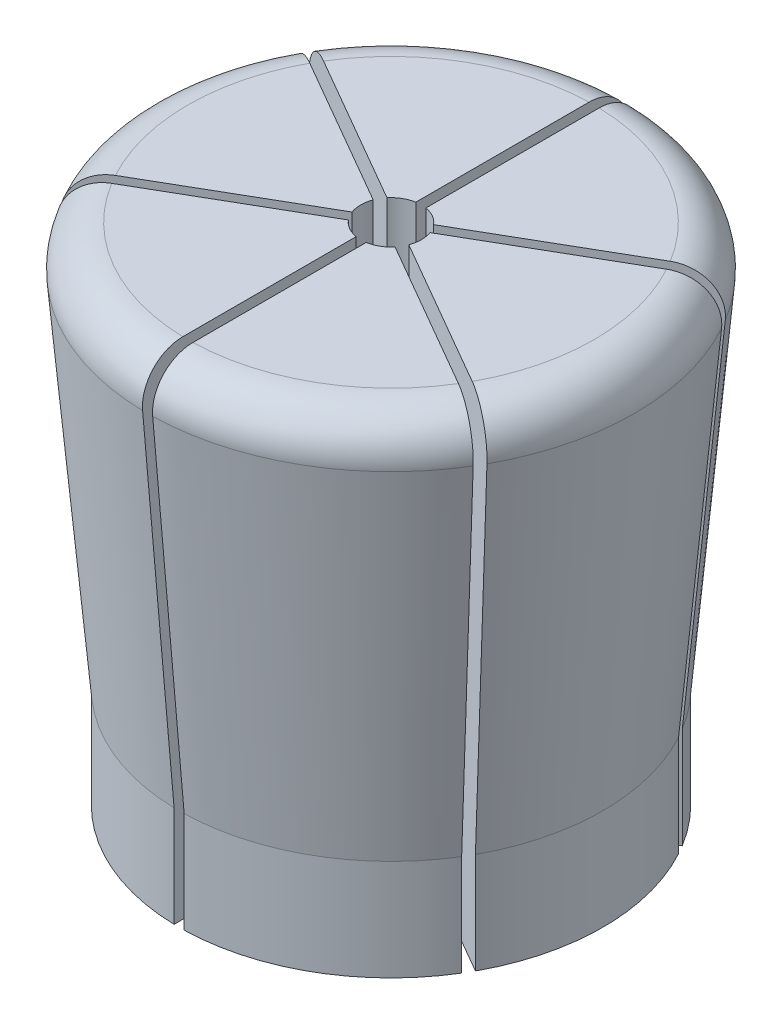
from build123d import *

# Parameters (mm, degrees)
SKETCH_2_R          = 1.5
CUT_EXTRUDE_1_DEPTH = 31.269333089
SKETCH_3_W          = 0.5
SKETCH_3_H          = 34.059940126
CUT_EXTRUDE_2_DEPTH = 31.269333089
CUT_EXTRUDE_3_DEPTH = 31.268300756
CUT_EXTRUDE_4_DEPTH = 31.268300756


with BuildPart() as part:
    # 草图1 → 旋转1 (revolve)
    with BuildSketch(Plane.XY, mode=Mode.PRIVATE) as revolve_1_sk:
        with BuildLine():
            Line((0, 25), (10.067156268, 25))
            ThreePointArc((10.067156268, 25), (11.541710942, 24.351180415), (12.059545665, 22.825688515))
            Line((12.059545665, 22.825688515), (10.5, 5))
            Line((10.5, 5), (10.5, 0))
            Line((10.5, 0), (0, 0))
            Line((0, 0), (0, 25))
        make_face()
    revolve(revolve_1_sk.sketch.rotate(Axis((0, 0, 0), (0, 1, 0)), 90), axis=Axis((0, 0, 0), (0, 1, 0)))

    # 草图2 → 切除-拉伸1 (cut, through all)
    with BuildSketch(Plane(origin=(0, 25, 0), x_dir=(1, 0, 0), z_dir=(0, 1, 0))):
        with Locations(Location((0, 0, 0), (0, 0, 270))):
            Circle(SKETCH_2_R)
    extrude(amount=-CUT_EXTRUDE_1_DEPTH, mode=Mode.SUBTRACT)

    # 草图3 → 切除-拉伸2 (cut, through all)
    with BuildSketch(Plane(origin=(0, 25, 0), x_dir=(1, 0, 0), z_dir=(0, 1, 0))):
        Rectangle(SKETCH_3_W, SKETCH_3_H)
    extrude(amount=-CUT_EXTRUDE_2_DEPTH, mode=Mode.SUBTRACT)


with BuildPart() as cut_extrude_2_piece_1:
    # of the separate pieces the step leaves, piece 1, a body of its own (cut_extrude_2_pieces)
    add(part.part.solids().sort_by_distance((0.25, 25, -10.064051636))[0])


with BuildPart() as cut_extrude_2_piece_2:
    # of the separate pieces the step leaves, piece 2, a body of its own (cut_extrude_2_pieces)
    add(part.part.solids().sort_by_distance((-0.25, 25, -10.064051636))[0])


with BuildPart() as cut_extrude_3_tool:
    # 草图4 → 切除-拉伸3 (new, through all)
    with BuildSketch(Plane(origin=(0, 25, 0), x_dir=(1, 0, 0), z_dir=(0, 1, 0))):
        Polygon((18.851057357, -11.172338174), (19.101057357, -10.739325472), (-18.851057357, 11.172338174), (-19.101057357, 10.739325472), align=None)
    extrude(amount=-CUT_EXTRUDE_3_DEPTH)


with BuildPart() as cut_extrude_2_piece_1_1:
    add(cut_extrude_2_piece_1.part)

    # 切除-拉伸3: cut by cut_extrude_3_tool
    add(cut_extrude_3_tool.part, mode=Mode.SUBTRACT)


with BuildPart() as cut_extrude_2_piece_2_1:
    add(cut_extrude_2_piece_2.part)

    # 切除-拉伸3: cut by cut_extrude_3_tool
    add(cut_extrude_3_tool.part, mode=Mode.SUBTRACT)


with BuildPart() as cut_extrude_3_piece_1:
    # of the separate pieces the step leaves, piece 1, a body of its own (cut_extrude_3_pieces)
    add(cut_extrude_2_piece_1_1.part.solids().sort_by_distance((0.25, 25, -10.064051636))[0])


with BuildPart() as cut_extrude_3_piece_2:
    # of the separate pieces the step leaves, piece 2, a body of its own (cut_extrude_3_pieces)
    add(cut_extrude_2_piece_1_1.part.solids().sort_by_distance((1.155868846, 25, 0.956016324))[0])


with BuildPart() as cut_extrude_3_piece_1_of_cut_extrude_2_p:
    # of the separate pieces the step leaves, piece 1, a body of its own (cut_extrude_3_pieces_of_cut_extrude_2_pi)
    add(cut_extrude_2_piece_2_1.part.solids().sort_by_distance((-8.840724382, 25, -4.815519467))[0])


with BuildPart() as cut_extrude_3_piece_2_of_cut_extrude_2_p:
    # of the separate pieces the step leaves, piece 2, a body of its own (cut_extrude_3_pieces_of_cut_extrude_2_pi)
    add(cut_extrude_2_piece_2_1.part.solids().sort_by_distance((-0.25, 25, -10.064051636))[0])


with BuildPart() as cut_extrude_4_tool:
    # 草图5 → 切除-拉伸4 (new, through all)
    with BuildSketch(Plane(origin=(0, 25, 0), x_dir=(1, 0, 0), z_dir=(0, 1, 0))):
        Polygon((-13.95064617, -7.765734187), (-13.70064617, -8.198746889), (13.95064617, 7.765734187), (13.70064617, 8.198746889), align=None)
    extrude(amount=-CUT_EXTRUDE_4_DEPTH)


with BuildPart() as cut_extrude_3_piece_1_1:
    add(cut_extrude_3_piece_1.part)

    # 切除-拉伸4: cut by cut_extrude_4_tool
    add(cut_extrude_4_tool.part, mode=Mode.SUBTRACT)


with BuildPart() as cut_extrude_3_piece_1_of_cut_extrude_2_p_1:
    add(cut_extrude_3_piece_1_of_cut_extrude_2_p.part)

    # 切除-拉伸4: cut by cut_extrude_4_tool
    add(cut_extrude_4_tool.part, mode=Mode.SUBTRACT)


with BuildPart() as cut_extrude_4_piece_1:
    # of the separate pieces the step leaves, piece 1, a body of its own (cut_extrude_4_pieces)
    add(cut_extrude_3_piece_1_1.part.solids().sort_by_distance((1.405868846, 25, -0.523003622))[0])


with BuildPart() as cut_extrude_4_piece_2:
    # of the separate pieces the step leaves, piece 2, a body of its own (cut_extrude_4_pieces)
    add(cut_extrude_3_piece_1_1.part.solids().sort_by_distance((0.25, 25, -10.064051636))[0])


with BuildPart() as cut_extrude_4_piece_1_of_cut_extrude_3_p:
    # of the separate pieces the step leaves, piece 1, a body of its own (cut_extrude_4_pieces_of_cut_extrude_3_pi)
    add(cut_extrude_3_piece_1_of_cut_extrude_2_p_1.part.solids().sort_by_distance((-8.840724382, 25, -4.815519467))[0])


with BuildPart() as cut_extrude_4_piece_2_of_cut_extrude_3_p:
    # of the separate pieces the step leaves, piece 2, a body of its own (cut_extrude_4_pieces_of_cut_extrude_3_pi)
    add(cut_extrude_3_piece_1_of_cut_extrude_2_p_1.part.solids().sort_by_distance((-8.590724382, 25, 5.248532169))[0])


solid = Compound([cut_extrude_3_piece_2.part, cut_extrude_3_piece_2_of_cut_extrude_2_p.part, cut_extrude_4_piece_1.part, cut_extrude_4_piece_2.part, cut_extrude_4_piece_1_of_cut_extrude_3_p.part, cut_extrude_4_piece_2_of_cut_extrude_3_p.part])
